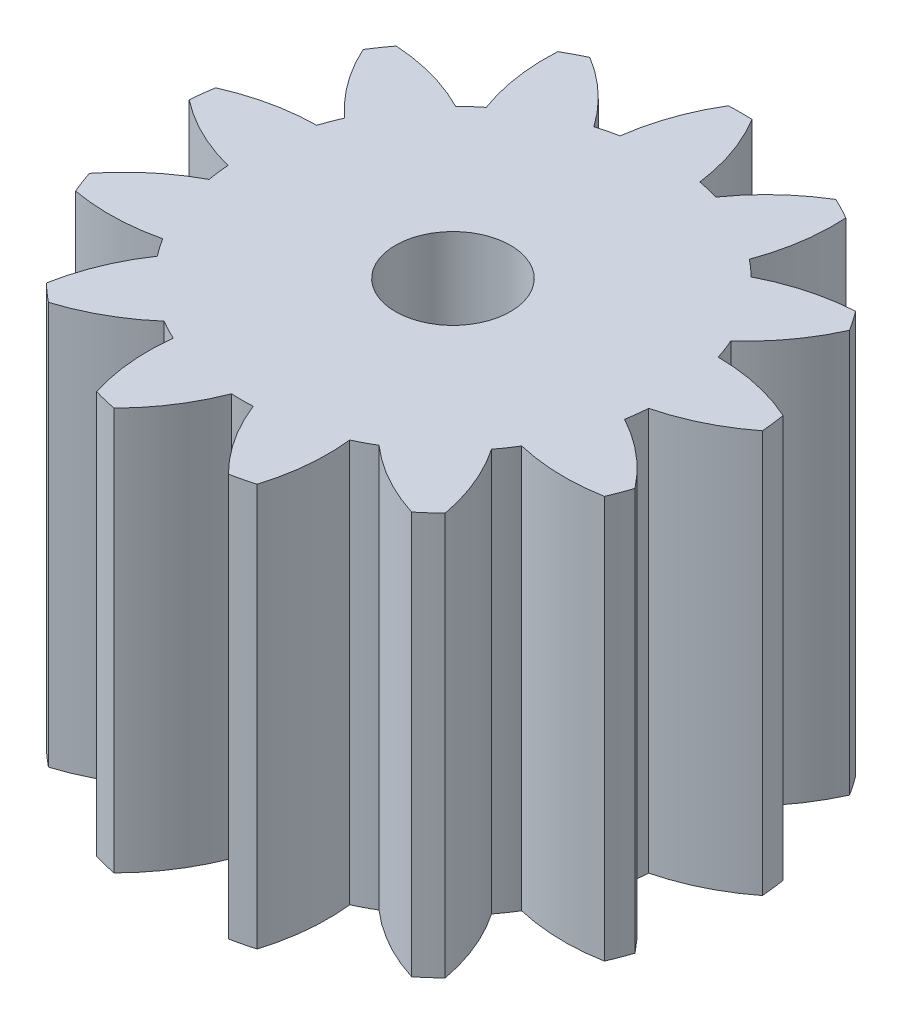
SolidWorks part; units mm, degrees
ref_plane "Front Plane" through (0, 0, 0) normal (0, 0, 1) x (1, 0, 0)
ref_plane "Top Plane" through (0, 0, 0) normal (0, 1, 0) x (1, 0, 0)
ref_plane "Right Plane" through (0, 0, 0) normal (1, 0, 0) x (0, 0, -1)
sketch "Sketch1" plane through (0, 0, 0) normal (0, 1, 0) x (1, 0, 0)
  line L0 (0, 0) -> (0, 10.3828) construction
  arc A0 (0.31, 7.4936) -> (-0.31, 7.4936) centre (0, 0) ccw
  circle A1 centre (0, 0) radius 5.5
  arc A2 (-1.04, 5.4008) -> (-0.31, 7.4936) centre (4.3152, 4.7065) cw
  arc A3 (1.04, 5.4008) -> (0.31, 7.4936) centre (-4.3152, 4.7065) ccw
  arc A4 (1.589, 5.2655) -> (3.208, 6.7793) centre (6.0081, 2.1621) cw
  arc A5 (3.4307, 4.2988) -> (3.7569, 6.4912) centre (-1.6337, 6.1728) ccw
  arc A6 (3.7569, 6.4912) -> (3.208, 6.7793) centre (0, 0) ccw
  arc A7 (3.854, 3.9239) -> (5.991, 4.512) centre (6.3247, -0.8777) cw
  arc A8 (5.0355, 2.2121) -> (6.3432, 4.0017) centre (1.4221, 6.225) ccw
  arc A9 (6.3432, 4.0017) -> (5.991, 4.512) centre (0, 0) ccw
  arc A10 (5.236, 1.6834) -> (7.4016, 1.211) centre (5.1924, -3.7164) cw
  arc A11 (5.4868, -0.3814) -> (7.4763, 0.5955) centre (4.1521, 4.851) ccw
  arc A12 (7.4763, 0.5955) -> (7.4016, 1.211) centre (0, 0) ccw
  arc A13 (5.4186, -0.9427) -> (7.1166, -2.3674) centre (2.8705, -5.7037) cw
  arc A14 (4.681, -2.8876) -> (6.8967, -2.9471) centre (5.9309, 2.3658) ccw
  arc A15 (6.8967, -2.9471) -> (7.1166, -2.3674) centre (0, 0) ccw
  arc A16 (4.3598, -3.3529) -> (5.2012, -5.4035) centre (-0.1089, -6.3844) cw
  arc A17 (2.8029, -4.7322) -> (4.7371, -5.8146) centre (6.351, -0.6614) ccw
  arc A18 (4.7371, -5.8146) -> (5.2012, -5.4035) centre (0, 0) ccw
  arc A19 (2.3023, -4.995) -> (2.0943, -7.2017) centre (-3.0634, -5.6025) cw
  arc A20 (0.2827, -5.4927) -> (1.4923, -7.35) centre (5.3161, -3.5371) ccw
  arc A21 (1.4923, -7.35) -> (2.0943, -7.2017) centre (0, 0) ccw
  arc A22 (-0.2827, -5.4927) -> (-1.4923, -7.35) centre (-5.3161, -3.5371) cw
  arc A23 (-2.3023, -4.995) -> (-2.0943, -7.2017) centre (3.0634, -5.6025) ccw
  arc A24 (-2.0943, -7.2017) -> (-1.4923, -7.35) centre (0, 0) ccw
  arc A25 (-2.8029, -4.7322) -> (-4.7371, -5.8146) centre (-6.351, -0.6614) cw
  arc A26 (-4.3598, -3.3529) -> (-5.2012, -5.4035) centre (0.1089, -6.3844) ccw
  arc A27 (-5.2012, -5.4035) -> (-4.7371, -5.8146) centre (0, 0) ccw
  arc A28 (-4.681, -2.8876) -> (-6.8967, -2.9471) centre (-5.9309, 2.3658) cw
  arc A29 (-5.4186, -0.9427) -> (-7.1166, -2.3674) centre (-2.8705, -5.7037) ccw
  arc A30 (-7.1166, -2.3674) -> (-6.8967, -2.9471) centre (0, 0) ccw
  arc A31 (-5.4868, -0.3814) -> (-7.4763, 0.5955) centre (-4.1521, 4.851) cw
  arc A32 (-5.236, 1.6834) -> (-7.4016, 1.211) centre (-5.1924, -3.7164) ccw
  arc A33 (-7.4016, 1.211) -> (-7.4763, 0.5955) centre (0, 0) ccw
  arc A34 (-5.0355, 2.2121) -> (-6.3432, 4.0017) centre (-1.4221, 6.225) cw
  arc A35 (-3.854, 3.9239) -> (-5.991, 4.512) centre (-6.3247, -0.8777) ccw
  arc A36 (-5.991, 4.512) -> (-6.3432, 4.0017) centre (0, 0) ccw
  arc A37 (-3.4307, 4.2988) -> (-3.7569, 6.4912) centre (1.6337, 6.1728) cw
  arc A38 (-1.589, 5.2655) -> (-3.208, 6.7793) centre (-6.0081, 2.1621) ccw
  arc A39 (-3.208, 6.7793) -> (-3.7569, 6.4912) centre (0, 0) ccw
  point P73 (0, 0)
  point P86 (0, 0)
  dimension "D1" = 15
  dimension "D2" = 11
  dimension "D5" = 5.4
  dimension "D3" = 0.62
  dimension "D4" = 2.08
  dimension "D6" = 13
extrude "Boss-Extrude1" add sketch "Sketch1" along normal blind 10.5
sketch "Sketch2" plane through (0, 10.5, 0) normal (0, 1, 0) x (1, 0, 0)
  circle A0 centre (0, 0) radius 1.5
  dimension "D1" = 3
extrude "Cut-Extrude1" cut sketch "Sketch2" against normal blind 10.5
